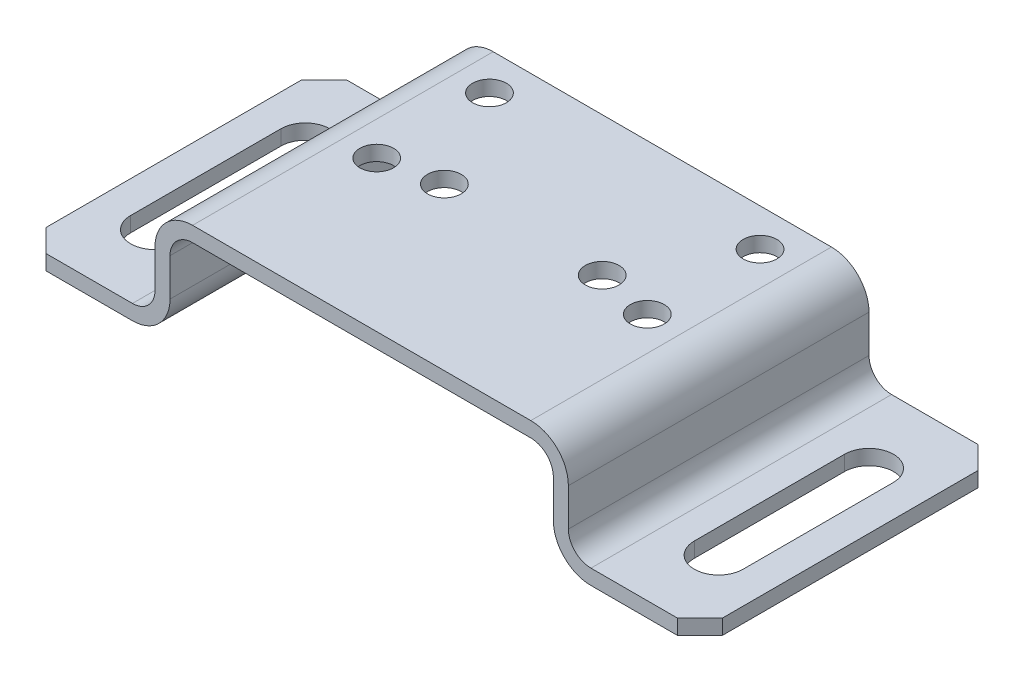
from build123d import *

# Parameters (mm, degrees)
EXTRUDE_1_DEPTH     = 40
CHAMFER_1_SIZE      = 3
CUT_EXTRUDE_1_DEPTH = 40
SKETCH_4_R          = 2.25
CUT_EXTRUDE_2_DEPTH = 40


with BuildPart() as part:
    # 草图2 → 凸台-拉伸1 (new body)
    with BuildSketch(Plane.XY):
        with BuildLine():
            Line((0, 0), (14.5, 0))
            ThreePointArc((14.5, 0), (16.621320344, 0.878679656), (17.5, 3))
            Line((17.5, 3), (17.5, 8))
            ThreePointArc((17.5, 8), (18.964466094, 11.535533906), (22.5, 13))
            Line((22.5, 13), (67.5, 13))
            ThreePointArc((67.5, 13), (71.035533906, 11.535533906), (72.5, 8))
            Line((72.5, 8), (72.5, 3))
            ThreePointArc((72.5, 3), (73.378679656, 0.878679656), (75.5, 0))
            Line((75.5, 0), (90, 0))
            Line((90, 0), (90, -2))
            Line((90, -2), (75.5, -2))
            ThreePointArc((75.5, -2), (71.964466094, -0.535533906), (70.5, 3))
            Line((70.5, 3), (70.5, 8))
            ThreePointArc((70.5, 8), (69.621320344, 10.121320344), (67.5, 11))
            Line((67.5, 11), (22.5, 11))
            ThreePointArc((22.5, 11), (20.378679656, 10.121320344), (19.5, 8))
            Line((19.5, 8), (19.5, 3))
            ThreePointArc((19.5, 3), (18.035533906, -0.535533906), (14.5, -2))
            Line((14.5, -2), (0, -2))
            Line((0, -2), (0, 0))
        make_face()
    extrude(amount=EXTRUDE_1_DEPTH)

    # 倒角1
    chamfer_1_edges = [part.edges().sort_by_distance(p)[0] for p in [
        (0, -1, 0),
        (90, -1, 0),
        (0, -1, 40),
        (90, -1, 40),
    ]]
    chamfer(chamfer_1_edges, length=CHAMFER_1_SIZE)

    # 草图3 → 切除-拉伸1 (cut)
    with BuildSketch(Plane(origin=(0, 0, 0), x_dir=(1, 0, 0), z_dir=(0, 1, 0))):
        with BuildLine():
            Line((4.25, -10), (4.25, -30))
            ThreePointArc((4.25, -30), (7.5, -33.25), (10.75, -30))
            Line((10.75, -30), (10.75, -10))
            ThreePointArc((10.75, -10), (7.5, -6.75), (4.25, -10))
        make_face()
        with BuildLine():
            ThreePointArc((85.75, -30), (82.5, -33.25), (79.25, -30))
            Line((79.25, -30), (79.25, -10))
            ThreePointArc((79.25, -10), (82.5, -6.75), (85.75, -10))
            Line((85.75, -10), (85.75, -30))
        make_face()
    extrude(amount=-CUT_EXTRUDE_1_DEPTH, mode=Mode.SUBTRACT)

    # 草图4 → 切除-拉伸2 (cut)
    with BuildSketch(Plane(origin=(0, 13, 0), x_dir=(1, 0, 0), z_dir=(0, 1, 0))):
        with Locations(Location((34.5, -18.5, 0), (0, 0, 270))):
            Circle(SKETCH_4_R)
        with Locations(Location((27, -20, 0), (0, 0, 270))):
            Circle(SKETCH_4_R)
        with Locations(Location((55.5, -18.5, 0), (0, 0, 270))):
            Circle(SKETCH_4_R)
        with Locations(Location((63, -20, 0), (0, 0, 270))):
            Circle(SKETCH_4_R)
        with Locations(Location((27, -5, 0), (0, 0, 270))):
            Circle(SKETCH_4_R)
        with Locations(Location((63, -5, 0), (0, 0, 270))):
            Circle(SKETCH_4_R)
    extrude(amount=-CUT_EXTRUDE_2_DEPTH, mode=Mode.SUBTRACT)


solid = part.part
